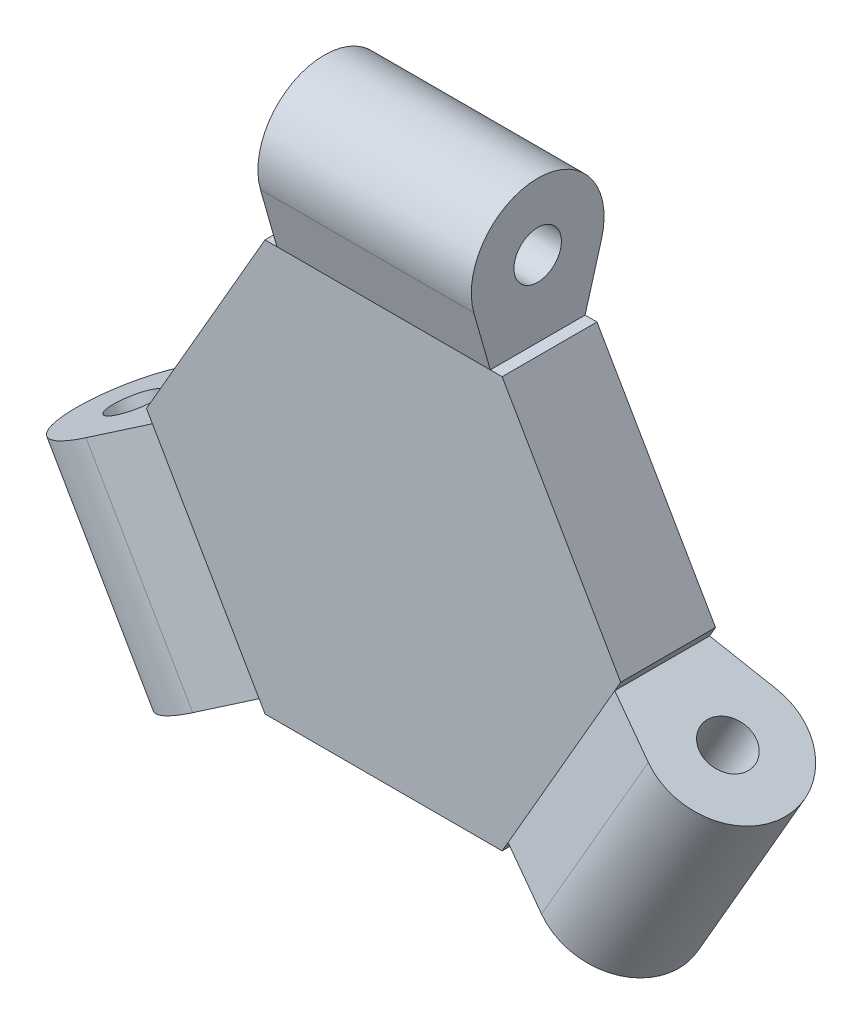
SolidWorks part; units mm, degrees
ref_plane "Front Plane" through (0, 0, 0) normal (0, 0, 1) x (1, 0, 0)
ref_plane "Top Plane" through (0, 0, 0) normal (0, 1, 0) x (1, 0, 0)
ref_plane "Right Plane" through (0, 0, 0) normal (1, 0, 0) x (0, 0, -1)
sketch "Sketch1" plane through (0, 0, 0) normal (0, 0, 1) x (1, 0, 0)
  line L1 (50, 0) -> (25, 43.3013)
  line L2 (25, 43.3013) -> (-25, 43.3013)
  line L3 (-25, 43.3013) -> (-50, 0)
  line L4 (-50, 0) -> (-25, -43.3013)
  line L5 (-25, -43.3013) -> (25, -43.3013)
  line L6 (25, -43.3013) -> (50, 0)
  circle A0 centre (0, 0) radius 43.3013 construction
  dimension "D1" = 50
extrude "Boss-Extrude1" add sketch "Sketch1" along normal blind 20
sketch "Sketch2" plane through (0, 0, 0) normal (1, 0, 0) x (0, 0, -1)
  line L0 (-20, 43.3013) -> (0, 43.3013) construction
  line L1 (-20, 43.3013) -> (-23.4651, 55.4659)
  line L2 (0, 43.3013) -> (3.4641, 55.4674)
  line L3 (-20, 0) -> (-20, 43.3013) construction
  line L4 (-20, 43.3013) -> (0, 43.3013)
  arc A0 (3.4641, 55.4674) -> (-23.4651, 55.4659) centre (-10.0007, 59.3013) ccw
  circle A1 centre (-10.0007, 59.3013) radius 5
  dimension "D1" = 28
  dimension "D2" = 16
  dimension "D4" = 10
  dimension "D3" = 9.9993
extrude "Boss-Extrude2" add sketch "Sketch2" along normal mid plane 45
sketch "Sketch4" plane through (0, 0, 0) normal (0, 0, -1) x (-1, 0, 0)
  circle A0 centre (0, 0) radius 5
  dimension "D1" = 10
extrude "Cut-Extrude1" cut sketch "Sketch4" against normal blind 0.5
pattern_circular "CirPattern1" count 3 over 360 about axis through (0, 0, 0) along (0, 0, 1) of "Boss-Extrude2"
